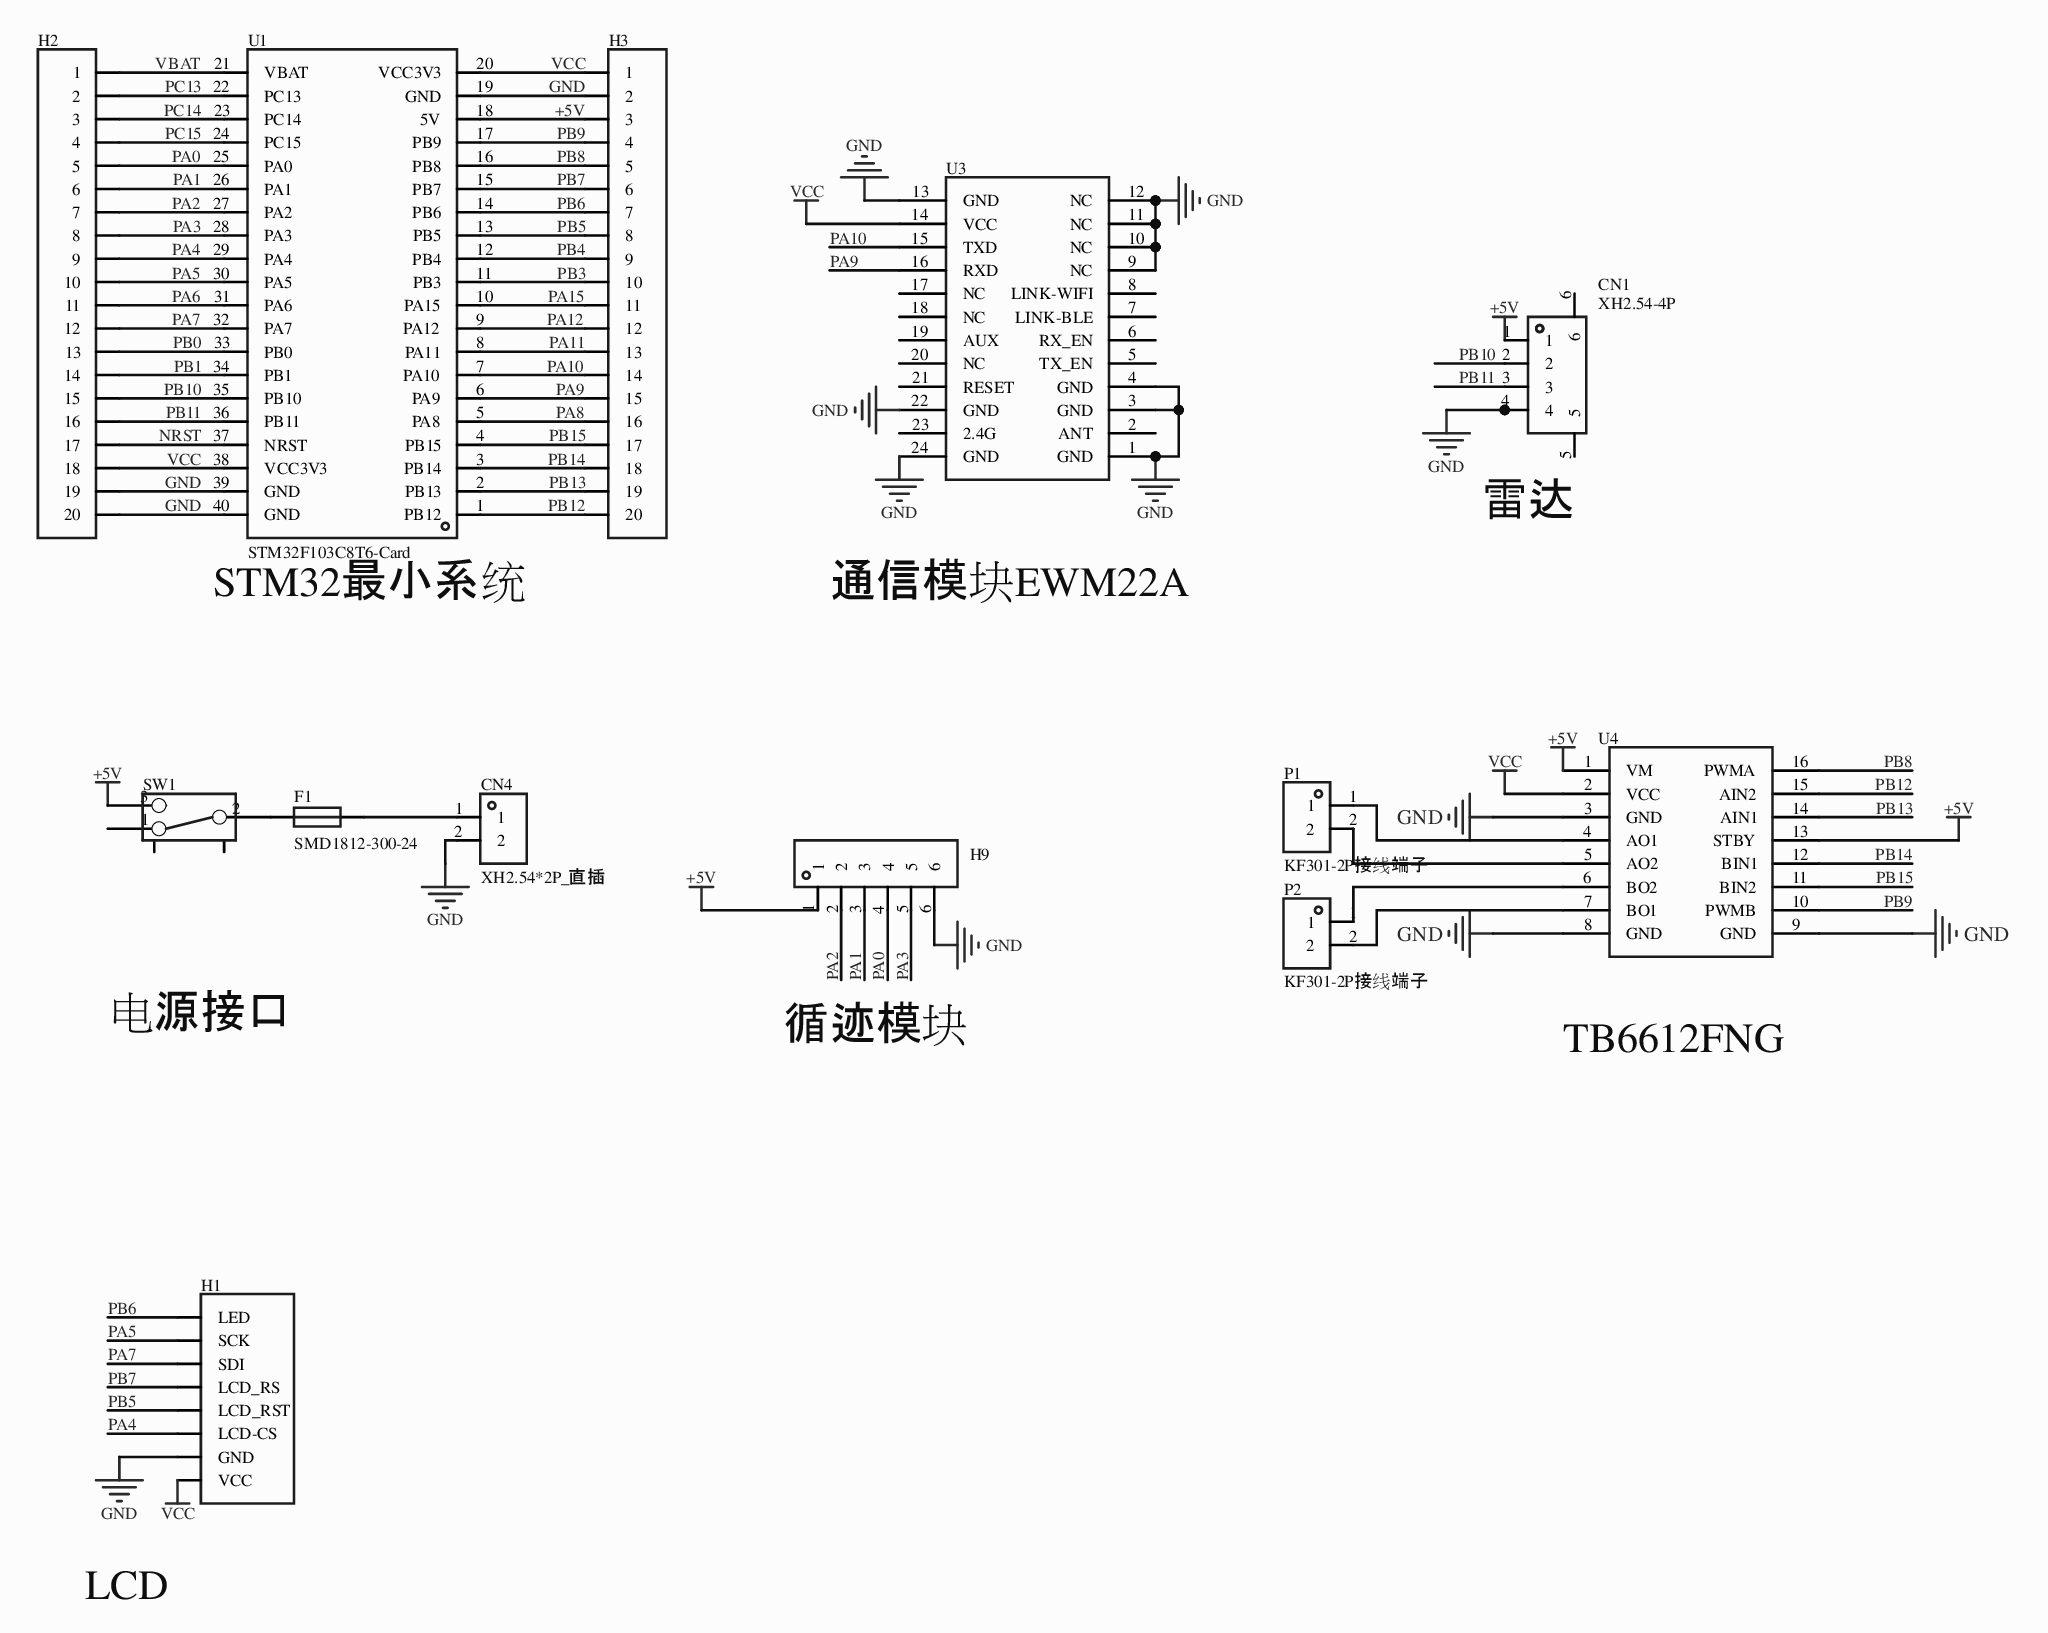
[diagram p0: MISC52128-3.schdoc]
# Altium project MISC52128-2.PrjPcb
1 sheet, 13 parts. Net scope: global (net labels, ports and power ports of the same name join across sheets).
Board file: MISC52128.pcbdoc

## Sheet MISC52128-3.schdoc
size 297 x 209 mm; Version: V1.0; @Project Name: MISC52128; @Page Count: 1; @Update Date: 2026-05-20; @Create Date: 2026-05-20; @Schematic Name: MISC52128; @Page No: 1; @Create Time: 23:22:16; @Update Time: 17:32:40; @Board Name: MISC52128

### Parts
CN1  XH2.54-4P  [CONN-SMD_4P-P2.50-WT]
CN4  XH2.54*2P_直插  [CONN-TH_2P-P2.50-XH2.54-2P]
F1  SMD1812-300-24  [F1812]
H1  (no value)  [HDR-TH_8P-P2.54-V-F-1]
H2  (no value)  [HDR-TH_20P-P2.54-V-F]
H3  (no value)  [HDR-TH_20P-P2.54-V-F]
H9  (no value)  [HDR-TH_6P-P2.54-V-F]
P1  KF301-2P接线端子  [CONN-TH_XY301V-A-5.0-2P]
P2  KF301-2P接线端子  [CONN-TH_XY301V-A-5.0-2P]
SW1  (no value)  [拨动开关_侧]
U1  STM32F103C8T6-Card  [CONN-TH_L53.3-W22.9_STM32F103C8T6-CARD]
U3  (no value)  [EWM22M-400/900T22S]
U4  (no value)  [tb6612]

### Nets
+5V: CN1.1 H3.3 H9.1 SW1.3 U1.18(5V) U4.1(VM) U4.13(STBY)
GND: CN1.4 CN4.2 H1.7(GND) H2.19 H2.20 H3.2 H9.6 U1.19(GND) U1.39(GND) U1.40(GND) U3.1(GND) U3.3(GND) U3.4(GND) U3.9(NC) U3.10(NC) U3.11(NC) U3.12(NC) U3.13(GND) U3.22(GND) U3.24(GND) U4.3(GND) U4.8(GND) U4.9(GND)
VCC: H1.8(VCC) H2.18 H3.1 U1.20(VCC3V3) U1.38(VCC3V3) U3.14(VCC) U4.2(VCC)
NRST: H2.17 U1.37(NRST)
PA0: H2.5 H9.4 U1.25(PA0)
PA1: H2.6 H9.3 U1.26(PA1)
PA2: H2.7 H9.2 U1.27(PA2)
PA3: H2.8 H9.5 U1.28(PA3)
PA4: H1.6(LCD-CS) H2.9 U1.29(PA4)
PA5: H1.2(SCK) H2.10 U1.30(PA5)
PA6: H2.11 U1.31(PA6)
PA7: H1.3(SDI) H2.12 U1.32(PA7)
PA8: H3.16 U1.5(PA8)
PA9: H3.15 U1.6(PA9) U3.16(RXD)
PA10: H3.14 U1.7(PA10) U3.15(TXD)
PA11: H3.13 U1.8(PA11)
PA12: H3.12 U1.9(PA12)
PA15: H3.11 U1.10(PA15)
PB0: H2.13 U1.33(PB0)
PB1: H2.14 U1.34(PB1)
PB3: H3.10 U1.11(PB3)
PB4: H3.9 U1.12(PB4)
PB5: H1.5(LCD_RST) H3.8 U1.13(PB5)
PB6: H1.1(LED) H3.7 U1.14(PB6)
PB7: H1.4(LCD_RS) H3.6 U1.15(PB7)
PB8: H3.5 U1.16(PB8) U4.16(PWMA)
PB9: H3.4 U1.17(PB9) U4.10(PWMB)
PB10: CN1.2 H2.15 U1.35(PB10)
PB11: CN1.3 H2.16 U1.36(PB11)
PB12: H3.20 U1.1(PB12) U4.15(AIN2)
PB13: H3.19 U1.2(PB13) U4.14(AIN1)
PB14: H3.18 U1.3(PB14) U4.12(BIN1)
PB15: H3.17 U1.4(PB15) U4.11(BIN2)
PC13: H2.2 U1.22(PC13)
PC14: H2.3 U1.23(PC14)
PC15: H2.4 U1.24(PC15)
VBAT: H2.1 U1.21(VBAT)
NetCN4_1: CN4.1 F1.2
NetF1_1: F1.1 SW1.2
NetP1_1: P1.1 U4.4(AO1)
NetP1_2: P1.2 U4.5(AO2)
NetP2_1: P2.1 U4.6(BO2)
NetP2_2: P2.2 U4.7(BO1)

Not connected (* = marked no-connect by the designer): CN1 5 6; SW1 1 4 5; U3 2(ANT) 5(TX_EN) 6(RX_EN) 7(LINK-BLE) 8(LINK-WIFI) 17(NC) 18(NC) 19(AUX) 20(NC) 21(RESET) 23(2.4G)

### Notes on the sheet
- (near CN1) 雷达
- (near U1) STM32最小系统
- 通信模块EWM22A
- 电源接口
- 循迹模块
- (near U4) TB6612FNG
- LCD

### Library data of the parts
CN1 = XH2.54-4P: Symbol: XH2.54-4P_C9900004347; AddInBom: yes; ModelId: 63317e43494a4a3ab58d4d70316633880819f05c4eef4c71ace90d822a990e87; ModelTransform: 590.55,393.7,0,0,0,0,0,-9.961,0; Device: XH2.54-4P; LCSC Part Name: XH2.54-4P; SupplierPart: C9900004347; ManufacturerPart: XH2.54-4P; Supplier Footprint: XH2.54-3PSMD; JLCPCB Part Class: Extended Part; Supplier: LCSC; ConvertToPcb: yes; FootprintName: CONN-SMD_4P-P2.50-WT; ModelName: CONN-SMD_4P-P2.50-WT
CN4 = XH2.54*2P_直插: AddInBom: yes; ModelId: 325c595e30db4df8abe76612dd40b0fa0819f05c4eef4c71ace90d822a990e87; ModelTransform: 295.275,228.346,0,180,0,0,-0.002,-20.079,-137.795; Device: XH2.54*2P_直插; Symbol: XH2.54*2P_直插; FootprintName: CONN-TH_2P-P2.50-XH2.54-2P; LCSC Part Name: XH2.54*2P_直插; SupplierPart: C9900008615; ManufacturerPart: XH2.54*2P_直插; Supplier Footprint: XH2.54_2P; JLCPCB Part Class: Extended Part; Supplier: LCSC; ConvertToPcb: yes; ModelName: CONN-TH_2P-P2.50-XH2.54-2P
F1 = SMD1812-300-24: 耐压(Vmax):24V;最大电流(Imax):40A;保持电流(Ihold):3A;跳闸电流(Itrip):6A;; Manufacturer: R+O(宏嘉诚); AddInBom: yes; ModelId: bca21e458c564d38b781621ca22e660b0819f05c4eef4c71ace90d822a990e87; ModelName: F1812_L4.5-W3.2-H1.0; ModelTransform: 177.165,125.984,0,0,0,0,0.0005,0,0; Voltage - Max: 24V; Current - Max: 40A; Hold Current: 3A; Trip Current: 6A; Power Dissipation: 1.4W; Resistance - Initial (Ri) (Min): 10mΩ; Resistance - Post Trip (R1) (Max): 50mΩ; Time to Trip(Max): 4s; Symbol: SMD1812-300-24; Device: SMD1812-300-24; LCSC Part Name: 24V 3A; SupplierPart: C49260581; ManufacturerPart: SMD1812-300-24; Supplier Footprint: 1812; JLCPCB Part Class: Extended Part; Datasheet: https://item.szlcsc.com/datasheet/SMD1812-300-24/51700394.html; Supplier: LCSC; ConvertToPcb: yes; FootprintName: F1812; Operating Temperature: -40℃~+85℃; Length: -; Width: -; Height: -; Pitch: -
H1 = HDR-F_2.54_1x8P: Symbol: Header-Female-2.54_1x8_2; AddInBom: yes; ModelId: 0f7e4d9227ef4fa08d5469c22cc70cdb; ModelName: HDR-F-2.54_1x8; ModelTransform: 799.99844,100,0,0,0,0,0,0,-118.11; Device: HDR-F_2.54_1x8P; ConvertToPcb: yes; FootprintName: HDR-TH_8P-P2.54-V-F-1; SupplierPart: C27438; Supplier Footprint: 插件
H2 H3 = HDR-F_2.54_1x20P: ConvertToPcb: yes; ModelId: db7015f7ad9d48b8a3b1188db02e3429; ModelName: HDR-F-2.54_1x20; ModelTransform: 1999.996,100,0,0,0,0,0,0,-118.11; Symbol: HDR-F_2.54_1x20P; Device: HDR-F_2.54_1x20P; AddInBom: yes; SupplierPart: C50984; Supplier Footprint: 插件; FootprintName: HDR-TH_20P-P2.54-V-F
H9 = HDR-F_2.54_1x6P: Symbol: Header-Female-2.54_1x6; 3D Model: 0f5bcf94dcda47d085f24cdca1696fe9; 3D Model Transform: 619.684,94.488,0,0,0,0,0,0,-125.984; ConvertToPcb: yes; Device: HDR-F_2.54_1x6P; Supplier Part: C40877; Supplier Footprint: 插件; AddInBom: yes; FootprintName: HDR-TH_6P-P2.54-V-F; ModelName: HDR-TH_6P-P2.54-V-F
P1 P2 = KF301-2P接线端子: 3D Model: ef7ead88b0f2448d904975b26718870f; 3D Model Transform: 417.322,299.212,0,0,0,0,11.811,-7.835,-157.48; AddInBom: yes; Symbol: KF301-2P接线端子; Device: KF301-2P接线端子; LCSC Part Name: KF301-2P接线端子; Supplier Part: C9900016950; Manufacturer Part: KF301-2P接线端子; Supplier Footprint: CK301-2P; Supplier: LCSC; ConvertToPcb: yes; FootprintName: CONN-TH_XY301V-A-5.0-2P; ModelName: CONN-TH_XY301V-A-5.0-2P
SW1 = 拨动开关_侧: Symbol: 拨动开关; ConvertToPcb: yes; ModelId: 10ea2cc5ba004a75b38812aadef1031f0819f05c4eef4c71ace90d822a990e87; ModelName: SW-TH_SK-12D07-VG3; ModelTransform: 337.98,287.46,295.24,0,0,0,0,-57,-110; Device: 拨动开关_侧; AddInBom: yes; Supplier Footprint: 插件; FootprintName: 拨动开关_侧
U1 = STM32F103C8T6-Card: AddInBom: yes; Device: STM32F103C8T6-Card; Symbol: STM32F103C8T6-CARD; FootprintName: CONN-TH_L53.3-W22.9_STM32F103C8T6-CARD; LCSC Part Name: STM32F103C8T6-Card; SupplierPart: C9900077949; ManufacturerPart: STM32F103C8T6-Card; Supplier Footprint: 插件; Supplier: LCSC; ConvertToPcb: yes
U3 = EWM22A-400BWL22S: AddInBom: yes; Symbol: EWM22A-400BWL22S; Device: EWM22A-400BWL22S; FootprintName: EWM22M-400/900T22S; ConvertToPcb: yes; Description: EWM22A-400BWL22S
U4 = tb6612: AddInBom: yes; Symbol: tb6612; Device: tb6612; JLCPCB Part Class: 扩展库; ConvertToPcb: yes; FootprintName: tb6612